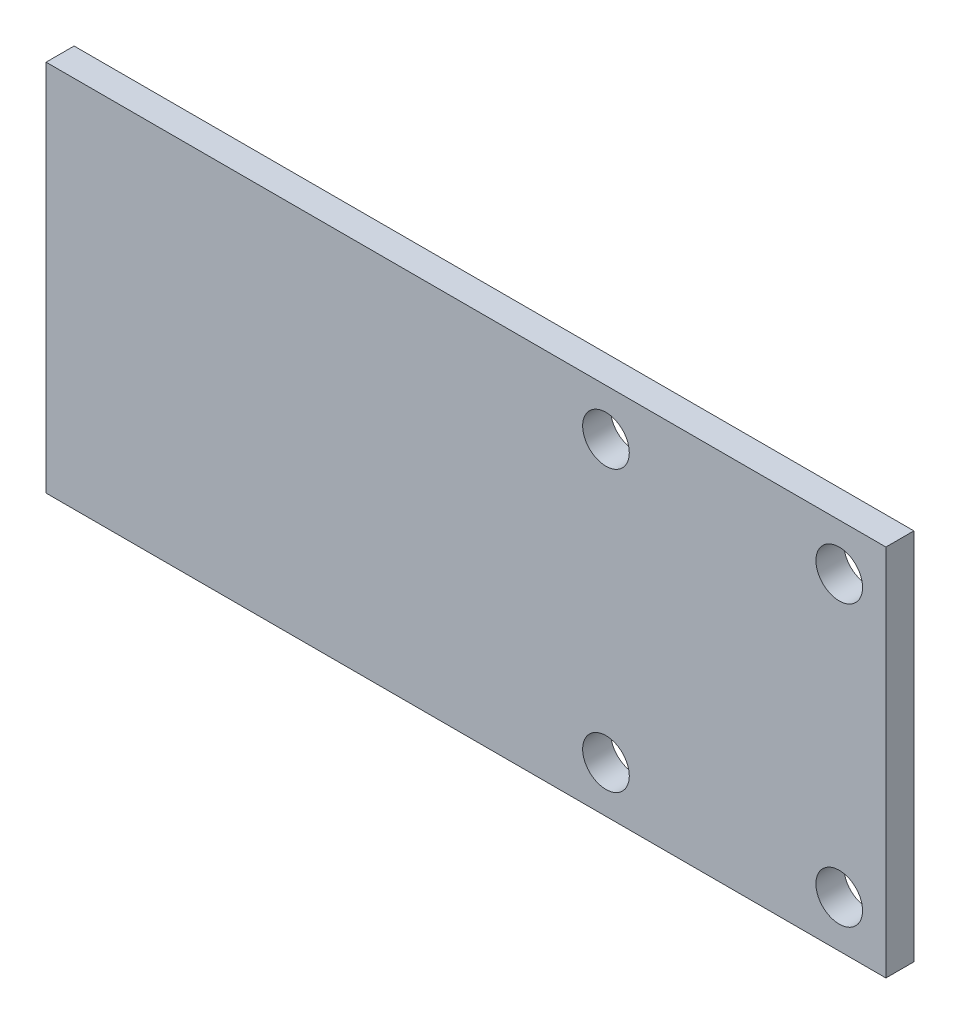
SolidWorks part; units mm, degrees
ref_plane "前视基准面" through (0, 0, 0) normal (0, 0, 1) x (1, 0, 0)
ref_plane "上视基准面" through (0, 0, 0) normal (0, 1, 0) x (1, 0, 0)
ref_plane "右视基准面" through (0, 0, 0) normal (1, 0, 0) x (0, 0, -1)
sketch "草图1" plane through (0, 0, 0) normal (0, 0, 1) x (1, 0, 0)
  line L0 (0, 0) -> (0, 80)
  line L1 (0, 80) -> (180, 80)
  line L2 (180, 80) -> (180, 0)
  line L3 (180, 0) -> (0, 0)
extrude "凸台-拉伸1" add sketch "草图1" along normal blind 6
sketch "草图2" plane through (0, 0, 6) normal (0, 0, 1) x (1, 0, 0)
  line L3 (180, 69.9987) -> (170, 69.9987)
  line L4 (180, 0) -> (180, 80) construction
  circle A4 centre (170, 69.9987) radius 5
  circle A5 centre (120, 9.9987) radius 5
  circle A6 centre (120, 69.9987) radius 5
  circle A7 centre (170, 9.9987) radius 5
extrude "切除-拉伸1" cut sketch "草图2" against normal blind 6
